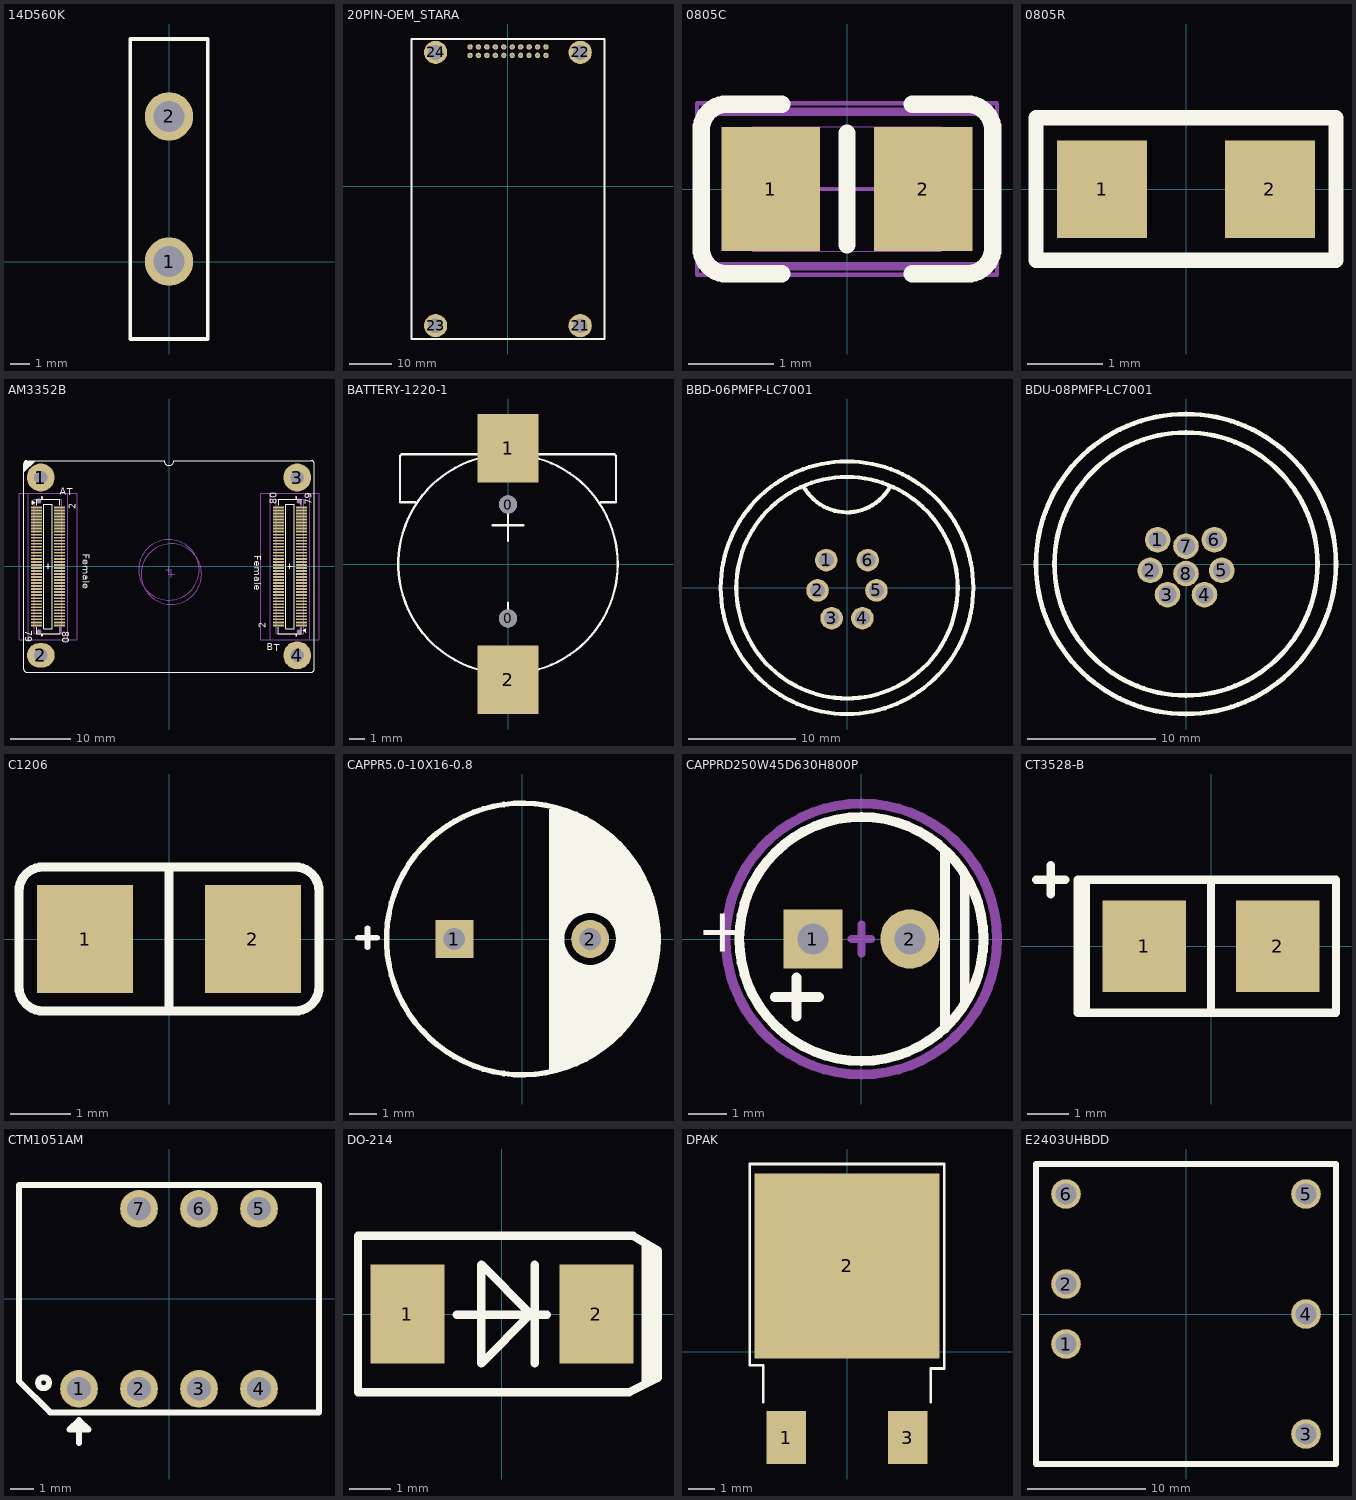
[diagram p0: the footprints below, top view; thin cyan lines are the x and y axes]
# Altium footprint library MISC84456-6.PcbLib: 41 footprints (part 1 of 3)
Each footprint in its own frame and in the unit in brackets; x right, y up, seen from the top. Pads: shape width x height; smd on the part's side, far side on the other; paste and mask are expansions set on the pad; w line width, h text height; cw(c..) or ccw(c..) is an arc to the next point about the centre after c.

## 14D560K [mm]
height 3.98
pads (2):
  round 2.5 hole 1.6: 1(0,0) 2(0,7.5)
Top Overlay:
  lines w0.2: -2,-4 -2,11.5 2,11.5 2,-4 -2,-4

## 20PIN-OEM_STARA [mm]
height 9.5
pads (24):
  round 1.3 hole 0.737: 1(-8.975,33.025) 2(-8.975,31.025) 3(-6.975,33.025) 4(-6.975,31.025) 5(-4.975,33.025) 6(-4.975,31.025) 7(-2.975,33.025) 8(-2.975,31.025) 9(-0.975,33.025) 11(1.025,33.025) 13(3.025,33.025) 15(5.025,33.025) 17(7.025,33.025) 19(9.025,33.025) 20(9.025,31.025)
  oval 1.2x1.3 hole 0.737: 10(-0.975,31.025) 12(1.025,31.025) 14(3.025,31.025) 16(5.025,31.025) 18(7.025,31.025)
  round 5.5 hole 3.5: 21(17.145,-33.025) 22(17.145,31.745) 23(-17.145,-33.025) 24(-17.145,31.745)
Top Overlay:
  lines w0.5: -22.805,-36.185 -22.805,34.915 22.855,34.915 22.855,-36.185 -22.805,-36.185

## 0805C [mm]
height 9.5
pads (2):
  rect 1.15x1.45 smd: 1(-0.889,0) 2(0.889,0)
Top Overlay:
  lines w0.2: 0,-0.65 0,0.65
  lines w0.203: -0.762,-0.991 -1.397,-0.991 cw(c-1.397,-0.686) -1.702,-0.686 -1.702,0.686 cw(c-1.397,0.686) -1.397,0.991 -0.762,0.991 ; 0.762,-0.991 1.397,-0.991 ccw(c1.397,-0.686) 1.702,-0.686 1.702,0.686 ccw(c1.397,0.686) 1.397,0.991 0.762,0.991
Mechanical 15:
  lines w0.1: -1.65,-0.9 -1.65,0.9 1.65,0.9 1.65,-0.9 -1.65,-0.9
  text "1" at -0.164,-0.45 h1.14
Mechanical 16:
  lines w0.001: -1.1,-0.725 -1.1,0.725 1.1,0.725 1.1,-0.725 -1.1,-0.725
  lines w0.05: -0.5,0 0.5,0 ; 0,-0.5 0,0.5 ; -1.75,-1 -1.75,1 1.75,1 1.75,-1 -1.75,-1
3D body: height 0.78, standoff 0, extent -1,-0.625 1,0.625

## 0805R [mm]
height 1.2
pads (2):
  rect 1.2x1.3 smd: 1(-1.118,0) 2(1.118,0)
Top Overlay:
  lines w0.203: -2,-0.95 -2,0.95 2,0.95 2,-0.95 -2,-0.95

## AM3352B [mm]
height 3.98
pads (172):
  round 0.6 hole 0.6 unplated mask+0.254: 0(-21.5,-10.8) 0(-21.5,-10.8) 0(-21.5,10.8) 0(-21.5,10.8) 0(21.5,-10.8) 0(21.5,-10.8) 0(21.5,10.8) 0(21.5,10.8)
  round 4.6 hole 2.2: 1(-21.2,14.7) 3(21.2,14.7) 4(21.2,-14.7)
  oval 4.6x4 hole 2.2: 2(-21.2,-14.7)
  rect 1.8x0.3 smd: A1(-21.9,9.75) A2(-18.1,9.75) A3(-21.9,9.25) A4(-18.1,9.25) A5(-21.9,8.75) A6(-18.1,8.75) A7(-21.9,8.25) A8(-18.1,8.25) A9(-21.9,7.75) A10(-18.1,7.75) A11(-21.9,7.25) A12(-18.1,7.25) A13(-21.9,6.75) A14(-18.1,6.75) A15(-21.9,6.25) A16(-18.1,6.25) A17(-21.9,5.75) A18(-18.1,5.75) A19(-21.9,5.25) A20(-18.1,5.25) A21(-21.9,4.75) A22(-18.1,4.75) A23(-21.9,4.25) A24(-18.1,4.25) A25(-21.9,3.75) A26(-18.1,3.75) A27(-21.9,3.25) A28(-18.1,3.25) A29(-21.9,2.75) A30(-18.1,2.75) A31(-21.9,2.25) A32(-18.1,2.25) A33(-21.9,1.75) A34(-18.1,1.75) A35(-21.9,1.25) A36(-18.1,1.25) A37(-21.9,0.75) A38(-18.1,0.75) A39(-21.9,0.25) A40(-18.1,0.25) A41(-21.9,-0.25) A42(-18.1,-0.25) A43(-21.9,-0.75) A44(-18.1,-0.75) A45(-21.9,-1.25) A46(-18.1,-1.25) A47(-21.9,-1.75) A48(-18.1,-1.75) A49(-21.9,-2.25) A50(-18.1,-2.25) A51(-21.9,-2.75) A52(-18.1,-2.75) A53(-21.9,-3.25) A54(-18.1,-3.25) A55(-21.9,-3.75) A56(-18.1,-3.75) A57(-21.9,-4.25) A58(-18.1,-4.25) A59(-21.9,-4.75) A60(-18.1,-4.75) A61(-21.9,-5.25) A62(-18.1,-5.25) A63(-21.9,-5.75) A64(-18.1,-5.75) A65(-21.9,-6.25) A66(-18.1,-6.25) A67(-21.9,-6.75) A68(-18.1,-6.75) A69(-21.9,-7.25) A70(-18.1,-7.25) A71(-21.9,-7.75) A72(-18.1,-7.75) A73(-21.9,-8.25) A74(-18.1,-8.25) A75(-21.9,-8.75) A76(-18.1,-8.75) A77(-21.9,-9.25) A78(-18.1,-9.25) A79(-21.9,-9.75) A80(-18.1,-9.75) B1(21.9,-9.75) B2(18.1,-9.75) B3(21.9,-9.25) B4(18.1,-9.25) B5(21.9,-8.75) B6(18.1,-8.75) B7(21.9,-8.25) B8(18.1,-8.25) B9(21.9,-7.75) B10(18.1,-7.75) B11(21.9,-7.25) B12(18.1,-7.25) B13(21.9,-6.75) B14(18.1,-6.75) B15(21.9,-6.25) B16(18.1,-6.25) B17(21.9,-5.75) B18(18.1,-5.75) B19(21.9,-5.25) B20(18.1,-5.25) B21(21.9,-4.75) B22(18.1,-4.75) B23(21.9,-4.25) B24(18.1,-4.25) B25(21.9,-3.75) B26(18.1,-3.75) B27(21.9,-3.25) B28(18.1,-3.25) B29(21.9,-2.75) B30(18.1,-2.75) B31(21.9,-2.25) B32(18.1,-2.25) B33(21.9,-1.75) B34(18.1,-1.75) B35(21.9,-1.25) B36(18.1,-1.25) B37(21.9,-0.75) B38(18.1,-0.75) B39(21.9,-0.25) B40(18.1,-0.25) B41(21.9,0.25) B42(18.1,0.25) B43(21.9,0.75) B44(18.1,0.75) B45(21.9,1.25) B46(18.1,1.25) B47(21.9,1.75) B48(18.1,1.75) B49(21.9,2.25) B50(18.1,2.25) B51(21.9,2.75) B52(18.1,2.75) B53(21.9,3.25) B54(18.1,3.25) B55(21.9,3.75) B56(18.1,3.75) B57(21.9,4.25) B58(18.1,4.25) B59(21.9,4.75) B60(18.1,4.75) B61(21.9,5.25) B62(18.1,5.25) B63(21.9,5.75) B64(18.1,5.75) B65(21.9,6.25) B66(18.1,6.25) B67(21.9,6.75) B68(18.1,6.75) B69(21.9,7.25) B70(18.1,7.25) B71(21.9,7.75) B72(18.1,7.75) B73(21.9,8.25) B74(18.1,8.25) B75(21.9,8.75) B76(18.1,8.75) B77(21.9,9.25) B78(18.1,9.25) B79(21.9,9.75) B80(18.1,9.75)
Top Overlay:
  circle w0.203: c-21.016,11.39 r0.102
  circle w0.203: c-21.016,-11.39 r0.102
  circle w0.203: c21.016,-11.39 r0.102
  circle w0.203: c21.016,11.39 r0.102
  region: -23.922,15.697 -22.195,17.424 -23.568,17.424 -23.922,17.069
  region: -22.159,10.566 -22.642,10.283 -22.642,10.85
  region: 22.159,-10.566 22.642,-10.282 22.642,-10.85
  lines w0.102: -24,-17 ccw(c-23.5,-17) -23.5,-17.5 23.5,-17.5 ccw(c23.5,-17) 24,-17 24,17 ccw(c23.5,17) 23.5,17.5 0.8,17.5 cw(c0,17.5) -0.8,17.5 -23.5,17.5 ccw(c-23.5,17) -24,17 -24,-17 ; -23.922,15.697 -23.922,16.924 cw(c-23.422,16.924) -23.422,17.424 -22.195,17.424 -23.922,15.697
  lines w0.127: -21.9,-10.084 -21.9,-11.1 -18.1,-11.1 -18.1,-10.084 ; -21.9,10.084 -21.9,11.1 -18.1,11.1 -18.1,10.084 ; 18.1,-10.084 18.1,-11.1 21.9,-11.1 21.9,-10.084 ; 18.1,10.084 18.1,11.1 21.9,11.1 21.9,10.084 ; -22.642,10.283 -22.159,10.566 -22.642,10.85 -22.642,10.283 ; -20.686,-10.3 -20.686,10.3 -19.314,10.3 -19.314,-10.3 -20.686,-10.3 ; 19.314,-10.3 20.686,-10.3 20.686,10.3 19.314,10.3 19.314,-10.3 ; 22.159,-10.566 22.642,-10.85 22.642,-10.282 22.159,-10.566
  lines w0.203: -20.4,0 -20,0 ; -20,-0.4 -20,0 ; -20,0.4 -20,0 ; -19.6,0 -20,0 ; 19.6,0 20,0 ; 20,-0.4 20,0 ; 20,0.4 20,0 ; 20.4,0 20,0
  text "T" at -15.951,11.735 h1.14
  text "80" at -17.628,-10.693 h1.14
  text "79" at -23.774,-10.566 h1.14
  text "2" at -15.443,9.423 h1.14
  text "Female" at -14.3,2.134 h1.14
  text "T" at 18.288,-13.995 h1.14
  text "80" at 17.78,10.262 h1.14
  text "79" at 23.597,10.211 h1.14
  text "2" at 15.977,-10.236 h1.14
  text "Female" at 14.122,1.829 h1.14
  text "A" at -18.059,11.836 h1.14
  text "B" at 16.18,-13.843 h1.14
Bottom Overlay:
  region: -22.083,10.566 -22.565,10.85 -22.565,10.283
  region: 22.083,-10.566 22.565,-10.85 22.565,-10.282
  region: -22.083,10.566 -22.565,10.85 -22.565,10.283
  lines w0.127: -22.565,10.283 -22.565,10.85 -22.083,10.566 -22.565,10.283 ; 22.083,-10.566 22.565,-10.85 22.565,-10.282 22.083,-10.566
Keep-Out Layer:
  circle w0.127: c21.5,10.8 r0.38
  circle w0.127: c21.5,-10.8 r0.38
  circle w0.127: c-21.5,-10.8 r0.38
  circle w0.127: c-21.5,-10.8 r0.38
  circle w0.127: c21.5,-10.8 r0.38
  circle w0.127: c-21.5,10.8 r0.38
  circle w0.127: c-21.5,10.8 r0.38
Mechanical 13:
  lines w0.152: -22.3,-11.1 -17.7,-11.1 -17.7,11.1 -22.3,11.1 -22.3,-11.1 ; 17.7,-11.1 17.7,11.1 22.3,11.1 22.3,-11.1 17.7,-11.1
Mechanical 15:
  lines w0.127: -20.432,0 -20,0 ; -20,-0.432 -20,0 ; -20,0.432 -20,0 ; -19.568,0 -20,0 ; 19.568,0 20,0 ; 20,-0.432 20,0 ; 20,0.432 20,0 ; 20.432,0 20,0
  lines w0.152: -23.3,-12.1 -23.3,12.1 ; -16.7,-12.1 -16.7,12.1 ; 16.7,-12.1 16.7,12.1 ; 23.3,-12.1 23.3,12.1 ; -24.8,-12.1 -24.8,12.1 -15.2,12.1 -15.2,-12.1 -24.8,-12.1 ; 15.2,-12.1 24.8,-12.1 24.8,12.1 15.2,12.1 15.2,-12.1
  text "元件禁布区" at -15.453,-3.353 h1.14
  text "元件禁布区" at -23.531,-3.353 h1.14
  text "元件禁布区" at 15.453,3.353 h1.14
  text "元件禁布区" at 23.531,3.353 h1.14
Mechanical 16:
  circle w0.001: c-0.017,-0.564 r5
  circle w0.001: c0.378,-1.264 r5
  lines w0.05: -0.517,-0.564 0.483,-0.564 ; -0.122,-1.264 0.878,-1.264 ; -0.017,-1.064 -0.017,-0.064 ; 0.378,-1.764 0.378,-0.764

## BATTERY-1220-1 [mm]
height 9.5
pads (4):
  round 1.2 hole 1.2: 0(0,-3.581) 0(0,3.912)
  rect 4x4.5 smd: 1(0,7.62) 2(0,-7.62)
Top Overlay:
  circle w0.152: c0,0 r7.22
  lines w0.152: -6.096,4.064 -7.112,4.064 -7.112,7.112 -7.004,7.22 0,7.22 7.004,7.22 7.112,7.112 7.112,4.064 6.096,4.064 ; -1.016,2.54 1.016,2.54 ; 0,-4.064 0,-2.54 ; 0,1.524 0,3.556

## BBD-06PMFP-LC7001 [mm]
pads (6):
  round 2.1 hole 1.4: 1(-1.93,2.56) 2(-2.74,-0.25) 3(-1.43,-2.84) 4(1.43,-2.84) 5(2.74,-0.25) 6(1.93,2.56)
Top Overlay:
  circle w0.381: c0,0 r11.75
  circle w0.381: c0,0 r10.3
  lines w0.381: -4.005,9.36 ccw(c-0.009,11.584) 3.937,9.271

## BDU-08PMFP-LC7001 [mm]
pads (8):
  round 2 hole 1.4: 1(-2.22,1.9) 2(-2.8,-0.5) 3(-1.45,-2.4) 4(1.45,-2.4) 5(2.8,-0.5) 6(2.22,1.9) 7(0,1.4) 8(0,-0.75)
Top Overlay:
  circle w0.381: c0,0 r11.75
  circle w0.381: c0,0 r10.3

## C1206 [mm]
pads (2):
  rect 1.6x1.8 smd: 1(-1.4,0) 2(1.4,0)
Top Overlay:
  lines w0.152: 0,-1.2 0,1.2 ; -2.5,-0.8 ccw(c-2.1,-0.8) -2.1,-1.2 2.1,-1.2 ccw(c2.1,-0.8) 2.5,-0.8 2.5,0.8 ccw(c2.1,0.8) 2.1,1.2 -2.1,1.2 ccw(c-2.1,0.8) -2.5,0.8 -2.5,-0.8
3D body: height 0.61, standoff 0, extent -1.524,-0.818 1.524,0.711

## CAPPR5.0-10X16-0.8 [mm]
height 3.98
pads (2):
  rect 1.4x1.4 hole 0.8: 1(-2.5,0)
  round 1.4 hole 0.8: 2(2.5,0)
Top Overlay:
  circle w0.5: c2.5,0 r1.2
  circle w0.203: c0,0 r5
  rectangle: 0.99,-4.815 1.39,4.785
  rectangle: 1.3,-4.7 1.5,4.8
  rectangle: 1.45,1 2.8,4.2
  rectangle: 2.7,1 3.5,3.6
  rectangle: 3.5,-3.2 3.8,3.3
  rectangle: 1.5,-3.5 3.5,-1
  rectangle: 1.5,-4.2 2.8,-3.3
  rectangle: 3.7,-2.6 4.2,2.8
  rectangle: 4.1,-1.8 4.6,2.2
  rectangle: 4.51,-1.085 4.91,1.415
  lines w0.203: -6.05,0.05 -5.7,0.05 ; -5.7,-0.3 -5.7,0.05 ; -5.7,0.4 -5.7,0.05 ; -5.35,0.05 -5.7,0.05
  lines w1: 1.514,-4.238 ccw(c0,0) 1.569,4.217
3D body: height 15.68, standoff -2.45, extent -5.1,-5.1 4.9,4.9

## CAPPRD250W45D630H800P [mm] "6.5mm"
height 8
pads (2):
  rect 1.524x1.524 hole 0.8: 1(-1.25,0)
  round 1.524 hole 0.8: 2(1.25,0)
Top Overlay:
  circle w0.254: c0,0 r3.15
  lines w0.254: -2.235,-1.499 -1.092,-1.499 ; -1.676,-2.007 -1.676,-0.991 ; 2.159,-2.311 2.159,2.261 ; 2.667,-1.676 2.667,1.626
  text "+" at -4.242,-0.33 h1.14
Mechanical 15:
  circle w0.254: c0,0 r3.5
  lines w0.203: -0.254,0 0,0 ; 0,-0.381 0,0 ; 0,0.381 0,0 ; 0.254,0 0,0
3D body: height 11.5, standoff -18.5, extent -3.15,-3.15 3.15,3.15

## CT3528-B [mm]
pads (2):
  rect 2x2.2 smd: 1(-1.6,0) 2(1.6,0)
Top Overlay:
  rectangle: -3.2,-1.5 -2.9,1.5
  lines w0.203: -4.2,1.6 -3.85,1.6 ; -3.85,1.25 -3.85,1.6 ; -3.85,1.95 -3.85,1.6 ; -3.5,1.6 -3.85,1.6 ; 0,-1.6 0,1.5 ; -3.2,-1.6 3,-1.6 3,1.6 -3.2,1.6 -3.2,-1.6
3D body: height 1.9, standoff 0, extent -1.75,-1.4 1.75,1.4

## CTM1051AM [mm] "7.7mm"
pads (7):
  round 1.6 hole 1: 1(-3.81,-3.81) 2(-1.27,-3.81) 3(1.27,-3.81) 4(3.81,-3.81) 5(3.81,3.81) 6(1.27,3.81) 7(-1.27,3.81)
Top Overlay:
  circle w0.254: c-5.31,-3.556 r0.23
  lines w0.254: -3.81,-6.096 -3.81,-5.131 ; -3.81,-5.131 -4.216,-5.537 -3.404,-5.537 -3.81,-5.131 ; -6.35,-3.489 -5.029,-4.81 6.35,-4.81 6.35,4.81 -6.35,4.81 -6.35,-3.489

## DO-214 [mm]
height 9.5
pads (2):
  rect 1.8x2.4 smd: 1(-2.3,0) 2(2.3,0)
Top Overlay:
  lines w0.203: -1.1,-0.02 1.1,-0.02 ; 0.8,-1.2 0.8,1.2 ; 3.5,-1.7 3.5,1.7 ; 3.7,-1.5 3.7,1.6 ; -3.5,-1.9 3.1,-1.9 3.8,-1.55 3.8,1.54 3.2,1.9 -3.5,1.9 -3.5,-1.9 ; -0.5,-1.2 0.7,0 -0.5,1.2 -0.5,-1.2

## DPAK [mm]
pads (3):
  rect 1.5x2 smd: 1(-2.3,-3.25) 3(2.3,-3.25)
  rect 7x7 smd: 2(0,3.25)
Top Overlay:
  lines w0.1: -3.175,-1.905 -3.175,-0.508 -3.683,-0.508 -3.683,6.858 -3.683,7.112 3.683,7.112 3.683,6.858 3.683,-0.635 3.175,-0.635 3.175,-1.905

## E2403UHBDD [mm]
height 9.5
pads (6):
  round 2.5 hole 1.8: 1(-10.16,-2.54) 2(-10.16,2.54) 3(10.16,-10.16) 4(10.16,0) 5(10.16,10.16) 6(-10.16,10.16)
Top Overlay:
  lines w0.5: -12.7,-12.7 12.7,-12.7 12.7,12.7 -12.7,12.7 -12.7,-12.7